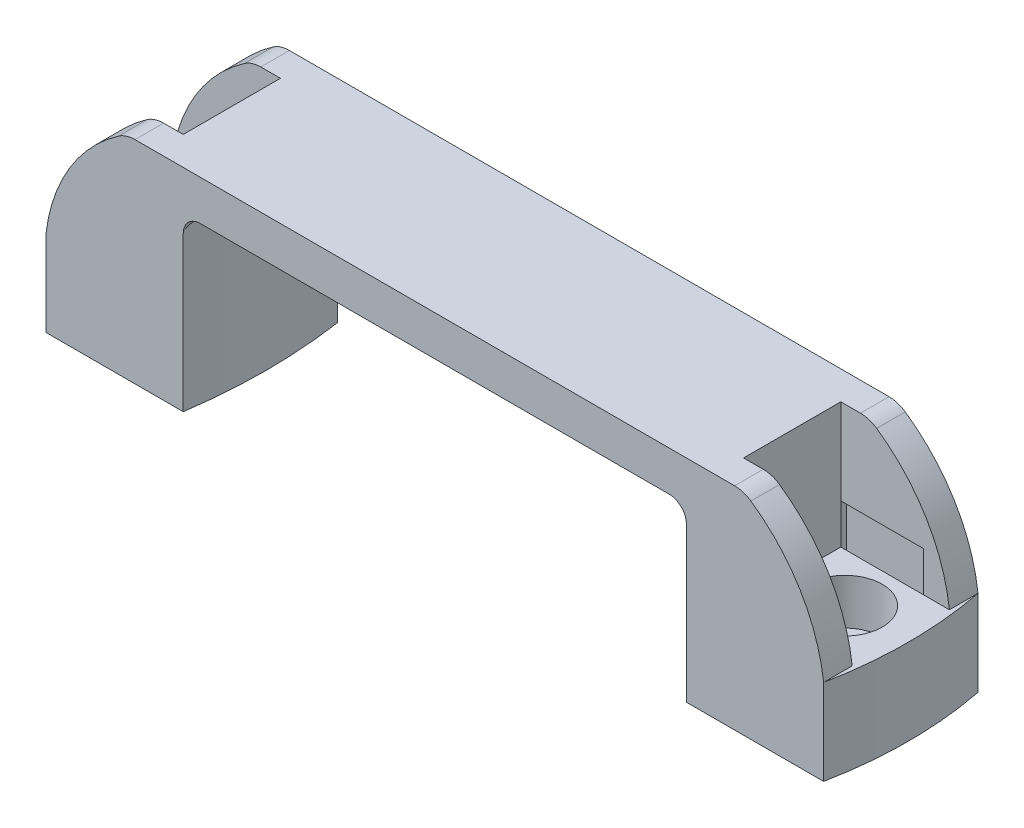
from build123d import *

# Parameters (mm, degrees)
EXTRUDE_1_DEPTH     = 13.5
EXTRUDE_2_REACH     = 80.583
EXTRUDE_3_DEPTH     = 15
CUT_EXTRUDE_1_DEPTH = 8.5
SKETCH_6_W          = 16
SKETCH_6_H          = 2.5
CUT_EXTRUDE_2_DEPTH = 22
SKETCH_7_R          = 6.5
CUT_EXTRUDE_3_DEPTH = 8
CUT_EXTRUDE_4_REACH = 78.737
SKETCH_8_R          = 4.1


with BuildPart() as part:
    # 草图1 → 凸台-拉伸1 (new, symmetric)
    with BuildSketch(Plane.XY):
        with BuildLine():
            Line((68, 0), (68, 15))
            ThreePointArc((68, 15), (63.909956901, 26.921785896), (55.283946786, 36.111420329))
            ThreePointArc((55.283946786, 36.111420329), (53.929013217, 36.772688008), (52.438560542, 37))
            Line((52.438560542, 37), (-52.438560542, 37))
            ThreePointArc((-52.438560542, 37), (-53.929013217, 36.772688008), (-55.283946786, 36.111420329))
            ThreePointArc((-55.283946786, 36.111420329), (-63.909956901, 26.921785896), (-68, 15))
            Line((-68, 15), (-68, 0))
            Line((-68, 0), (-44, 0))
            Line((-44, 0), (-44, 27))
            ThreePointArc((-44, 27), (-43.121320344, 29.121320344), (-41, 30))
            Line((-41, 30), (41, 30))
            ThreePointArc((41, 30), (43.121320344, 29.121320344), (44, 27))
            Line((44, 27), (44, 0))
            Line((44, 0), (68, 0))
        make_face()
    extrude(amount=EXTRUDE_1_DEPTH, both=True)

    # 凸台-拉伸2: up to this face of the body (flat: up to its plane)
    extrude_2_end = Plane(part.part.faces().sort_by_distance((0, 30, 0))[0])
    # 草图2 → 凸台-拉伸2 (add, up to the picked face)
    with BuildSketch(Plane.XZ, mode=Mode.PRIVATE) as extrude_2_sk1:
        with BuildLine():
            Line((-44, 13.5), (-44, -13.5))
            ThreePointArc((-44, -13.5), (-43, 0), (-44, 13.5))
        make_face()
    extrude_2_tool1 = split(extrude(extrude_2_sk1.sketch, amount=-EXTRUDE_2_REACH, mode=Mode.PRIVATE), bisect_by=extrude_2_end, keep=Keep.BOTH, mode=Mode.PRIVATE)
    # 草图2 → 凸台-拉伸2 (add, up to the picked face)
    with BuildSketch(Plane.XZ, mode=Mode.PRIVATE) as extrude_2_sk2:
        with BuildLine():
            Line((44, 13.5), (44, -13.5))
            ThreePointArc((44, -13.5), (43, 0), (44, 13.5))
        make_face()
    extrude_2_tool2 = split(extrude(extrude_2_sk2.sketch, amount=-EXTRUDE_2_REACH, mode=Mode.PRIVATE), bisect_by=extrude_2_end, keep=Keep.BOTH, mode=Mode.PRIVATE)
    add(extrude_2_tool1.solids().sort_by(Axis((-43.599812, 0, 0), (0, 1, 0)))[0])
    add(extrude_2_tool2.solids().sort_by(Axis((43.599812, 0, 0), (0, 1, 0)))[0])

    # 草图4 → 凸台-拉伸3 (add)
    with BuildSketch(Plane.XZ):
        with BuildLine():
            Line((-68, 13.5), (-68, -13.5))
            ThreePointArc((-68, -13.5), (-69.327123119, 0), (-68, 13.5))
        make_face()
        with BuildLine():
            Line((68, 13.5), (68, -13.5))
            ThreePointArc((68, -13.5), (69.327123119, 0), (68, 13.5))
        make_face()
    extrude(amount=-EXTRUDE_3_DEPTH)

    # 草图5 → 切除-拉伸1 (cut, symmetric)
    with BuildSketch(Plane.XY):
        with BuildLine():
            ThreePointArc((-52.438560542, 37), (-53.929013217, 36.772688008), (-55.283946786, 36.111420329))
            ThreePointArc((-55.283946786, 36.111420329), (-63.909956901, 26.921785896), (-68, 15))
            Line((-68, 15), (-49, 15))
            Line((-49, 15), (-49, 37))
            Line((-49, 37), (-52.438560542, 37))
        make_face()
        with BuildLine():
            ThreePointArc((52.438560542, 37), (53.929013217, 36.772688008), (55.283946786, 36.111420329))
            ThreePointArc((55.283946786, 36.111420329), (63.909956901, 26.921785896), (68, 15))
            Line((68, 15), (49, 15))
            Line((49, 15), (49, 37))
            Line((49, 37), (52.438560542, 37))
        make_face()
    extrude(amount=CUT_EXTRUDE_1_DEPTH, both=True, mode=Mode.SUBTRACT)

    # 草图6 → 切除-拉伸2 (cut)
    with BuildSketch(Plane.XZ):
        with Locations((-55.5, 9.75)):
            Rectangle(SKETCH_6_W, SKETCH_6_H)
        with Locations((55.5, 9.75)):
            Rectangle(SKETCH_6_W, SKETCH_6_H)
        with Locations((55.5, -9.75)):
            Rectangle(SKETCH_6_W, SKETCH_6_H)
        with Locations((-55.5, -9.75)):
            Rectangle(SKETCH_6_W, SKETCH_6_H)
    extrude(amount=-CUT_EXTRUDE_2_DEPTH, mode=Mode.SUBTRACT)

    # 草图7 → 切除-拉伸3 (cut)
    with BuildSketch(Plane(origin=(0, 15, 0), x_dir=(1, 0, 0), z_dir=(0, 1, 0))):
        with Locations(Location((-58.25, 0, 0), (0, 0, 180))):
            Circle(SKETCH_7_R)
        with Locations(Location((58.25, 0, 0), (0, 0, 180))):
            Circle(SKETCH_7_R)
    extrude(amount=-CUT_EXTRUDE_3_DEPTH, mode=Mode.SUBTRACT)

    # 草图8 → 切除-拉伸4 (cut, up to next)
    with BuildSketch(Plane(origin=(0, 7, 0), x_dir=(1, 0, 0), z_dir=(0, 1, 0)), mode=Mode.PRIVATE) as cut_extrude_4_sk1:
        with Locations(Location((58.25, 0, 0), (0, 0, 180))):
            Circle(SKETCH_8_R)
    cut_extrude_4_tool1 = extrude(cut_extrude_4_sk1.sketch, amount=-CUT_EXTRUDE_4_REACH, mode=Mode.PRIVATE) & part.part
    # 草图8 → 切除-拉伸4 (cut, up to next)
    with BuildSketch(Plane(origin=(0, 7, 0), x_dir=(1, 0, 0), z_dir=(0, 1, 0)), mode=Mode.PRIVATE) as cut_extrude_4_sk2:
        with Locations(Location((-58.25, 0, 0), (0, 0, 180))):
            Circle(SKETCH_8_R)
    cut_extrude_4_tool2 = extrude(cut_extrude_4_sk2.sketch, amount=-CUT_EXTRUDE_4_REACH, mode=Mode.PRIVATE) & part.part
    add(cut_extrude_4_tool1.solids().sort_by_distance((58.25, 7, 0))[0], mode=Mode.SUBTRACT)
    add(cut_extrude_4_tool2.solids().sort_by_distance((-58.25, 7, 0))[0], mode=Mode.SUBTRACT)


solid = part.part
